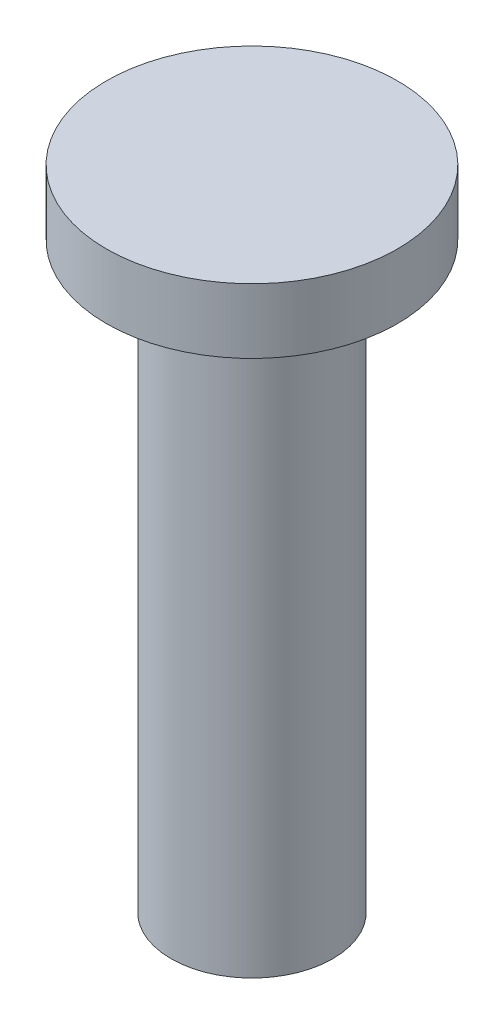
from build123d import *

# Parameters (mm, degrees)
SKETCH1_R           = 12.5
BOSS_EXTRUDE1_DEPTH = 100
SKETCH2_R           = 22.5
BOSS_EXTRUDE2_DEPTH = 10


with BuildPart() as part:
    # Sketch1 → Boss-Extrude1 (new body)
    with BuildSketch(Plane(origin=(0, 0, 0), x_dir=(1, 0, 0), z_dir=(0, 1, 0))):
        with Locations(Location((0, 0, 0), (0, 0, 270))):
            Circle(SKETCH1_R)
    extrude(amount=BOSS_EXTRUDE1_DEPTH)

    # Sketch2 → Boss-Extrude2 (add)
    with BuildSketch(Plane(origin=(0, 100, 0), x_dir=(1, 0, 0), z_dir=(0, 1, 0))):
        with Locations(Location((0, 0, 0), (0, 0, 270))):
            Circle(SKETCH2_R)
    extrude(amount=-BOSS_EXTRUDE2_DEPTH)


solid = part.part
